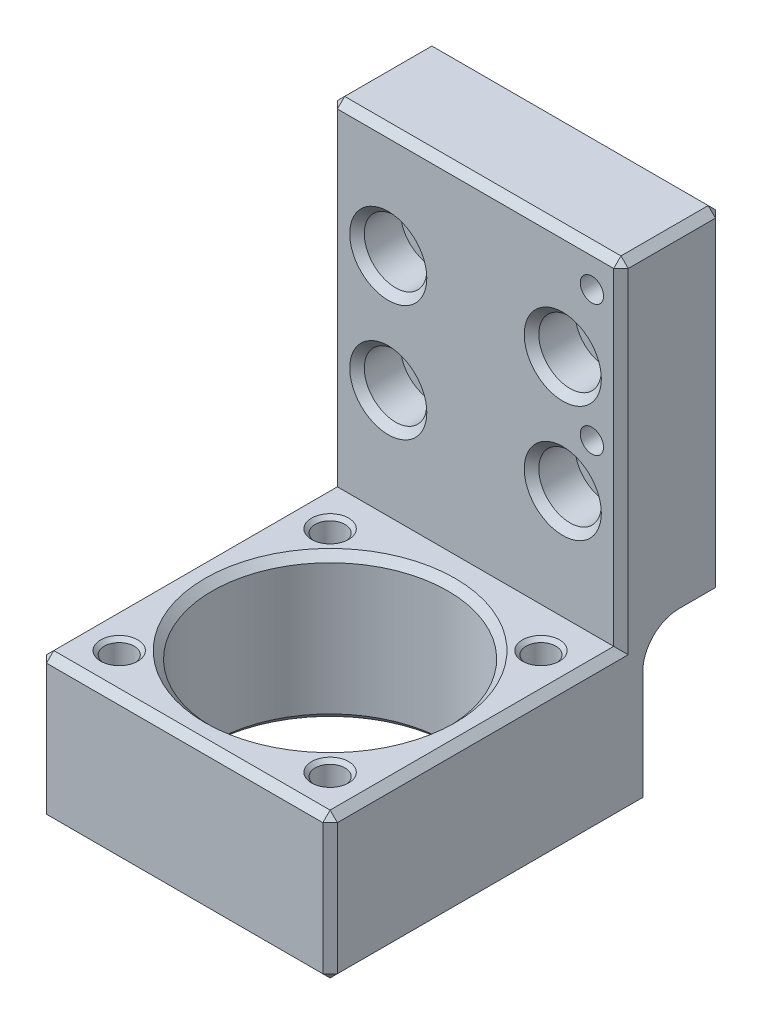
from build123d import *

# Parameters (mm, degrees)
BOSS_EXTRUDE1_DEPTH                                = 10
SKETCH2_R                                          = 8.1
CUT_EXTRUDE1_DEPTH                                 = 10
M2_5_TAPPED_HOLE1_D                                = 2.05
M2_5_TAPPED_HOLE1_DEPTH                            = 7.35
M2_5_TAPPED_HOLE1_CSINK_D                          = 2.55
M2_5_TAPPED_HOLE1_CSINK_ANGLE                      = 90
M2_5_TAPPED_HOLE1_TIP                              = 0.615882135
HOLE_SIZE_SOCKET_HEAD_CAP_SCREW_TYPE_0_D           = 2.4
HOLE_SIZE_SOCKET_HEAD_CAP_SCREW_TYPE_0_CBORE_D     = 4.3
HOLE_SIZE_SOCKET_HEAD_CAP_SCREW_TYPE_0_CBORE_DEPTH = 3
SKETCH9_W                                          = 5
SKETCH9_H                                          = 10
CUT_EXTRUDE4_DEPTH                                 = 6
M2_TAPPED_HOLE1_D                                  = 1.6
M2_TAPPED_HOLE1_DEPTH                              = 5.2
M2_TAPPED_HOLE1_TIP                                = 0.480688495
FILLET1_R                                          = 2
CHAMFER1_SIZE                                      = 0.5
M2_5_TAPPED_HOLE2_D                                = 2.05
M2_5_TAPPED_HOLE2_DEPTH                            = 6.35
M2_5_TAPPED_HOLE2_TIP                              = 0.615882135
M2_TAPPED_HOLE2_D                                  = 1.6


with BuildPart() as part:
    # Sketch1 → Boss-Extrude1 (new, symmetric)
    with BuildSketch(Plane(origin=(0, 0, 0), x_dir=(0, 0, -1), z_dir=(1, 0, 0))):
        Polygon((0, 33), (0, 0), (-27, 0), (-27, 10), (-7, 10), (-7, 33), align=None)
    extrude(amount=BOSS_EXTRUDE1_DEPTH, both=True)

    # Sketch2 → Cut-Extrude1 (cut)
    with BuildSketch(Plane(origin=(0, 10, 0), x_dir=(1, 0, 0), z_dir=(0, 1, 0))):
        with Locations(Location((0, -17, 0), (0, 0, 270))):
            Circle(SKETCH2_R)
    extrude(amount=-CUT_EXTRUDE1_DEPTH, mode=Mode.SUBTRACT)

    # M2.5 Tapped Hole1
    with Locations(Plane(origin=(0, 10, 0), x_dir=(1, 0, 0), z_dir=(0, 1, 0))):
        with Locations((-7.25, -9.75), (-7.25, -24.25), (7.25, -24.25), (7.25, -9.75)):
            CounterSinkHole(M2_5_TAPPED_HOLE1_D / 2, M2_5_TAPPED_HOLE1_CSINK_D / 2, depth=M2_5_TAPPED_HOLE1_DEPTH, counter_sink_angle=M2_5_TAPPED_HOLE1_CSINK_ANGLE)
            with Locations((0, 0, -(M2_5_TAPPED_HOLE1_DEPTH + M2_5_TAPPED_HOLE1_TIP / 2))):  # 118° drill point
                Cone(0, M2_5_TAPPED_HOLE1_D / 2, M2_5_TAPPED_HOLE1_TIP, mode=Mode.SUBTRACT)

    # Hole size socket head cap screw type 0 (through all)
    with Locations(Plane.XY.offset(7)):
        with Locations((-6, 25.5), (6, 25.5), (6, 17.5), (-6, 17.5)):
            CounterBoreHole(HOLE_SIZE_SOCKET_HEAD_CAP_SCREW_TYPE_0_D / 2, HOLE_SIZE_SOCKET_HEAD_CAP_SCREW_TYPE_0_CBORE_D / 2, HOLE_SIZE_SOCKET_HEAD_CAP_SCREW_TYPE_0_CBORE_DEPTH)

    # Sketch9 → Cut-Extrude4 (cut)
    with BuildSketch(Plane.ZY.offset(-10)):
        with Locations((2.5, 5)):
            Rectangle(SKETCH9_W, SKETCH9_H)
    extrude(amount=CUT_EXTRUDE4_DEPTH, mode=Mode.SUBTRACT)

    # M2 Tapped Hole1
    with Locations(Plane(origin=(4, 0, 0), x_dir=(0, 0, -1), z_dir=(1, 0, 0))):
        with Locations((-2.5, 7.5), (-2.5, 2.5)):
            Hole(M2_TAPPED_HOLE1_D / 2, depth=M2_TAPPED_HOLE1_DEPTH)
            with Locations((0, 0, -(M2_TAPPED_HOLE1_DEPTH + M2_TAPPED_HOLE1_TIP / 2))):  # 118° drill point
                Cone(0, M2_TAPPED_HOLE1_D / 2, M2_TAPPED_HOLE1_TIP, mode=Mode.SUBTRACT)

    # Fillet1
    fillet1_edges = [part.edges().sort_by_distance(p)[0] for p in [
        (7, 10, 5),
    ]]
    fillet(fillet1_edges, radius=FILLET1_R)

    # Chamfer1
    chamfer1_edges = [part.edges().sort_by_distance(p)[0] for p in [
        (10, 10, 1.5),
        (10, 9.414213562, 4.414213562),
        (0, 33, 0),
        (0, 0, 27),
        (0, 10, 27),
        (0, 33, 7),
        (10, 10, 17),
        (10, 5, 27),
        (0, 0, 8.9),
        (0, 10, 8.9),
        (10, 0, 16),
        (10, 33, 3.5),
        (-8.15, 17.5, 7),
        (-4.8, 17.5, 0),
        (3.85, 17.5, 7),
        (7.2, 17.5, 0),
        (3.85, 25.5, 7),
        (7.2, 25.5, 0),
        (-10, 16.5, 0),
        (-8.15, 25.5, 7),
        (-4.8, 25.5, 0),
        (-10, 0, 13.5),
        (-10, 5, 27),
        (10, 21.5, 0),
        (-10, 10, 17),
        (-3, 0, 0),
        (7, 10, 0),
        (10, 4, 5),
        (-10, 21.5, 7),
        (7, 0, 5),
        (-10, 33, 3.5),
        (10, 21.5, 7),
    ]]
    chamfer(chamfer1_edges, length=CHAMFER1_SIZE)

    # M2.5 Tapped Hole2
    with Locations(Plane.ZY.offset(10)):
        with Locations((3, 6)):
            Hole(M2_5_TAPPED_HOLE2_D / 2, depth=M2_5_TAPPED_HOLE2_DEPTH)
            with Locations((0, 0, -(M2_5_TAPPED_HOLE2_DEPTH + M2_5_TAPPED_HOLE2_TIP / 2))):  # 118° drill point
                Cone(0, M2_5_TAPPED_HOLE2_D / 2, M2_5_TAPPED_HOLE2_TIP, mode=Mode.SUBTRACT)

    # M2 Tapped Hole2 (through all)
    with Locations(Plane.XY.offset(7)):
        with Locations((8, 30.5), (8, 21.5)):
            Hole(M2_TAPPED_HOLE2_D / 2)


solid = part.part
